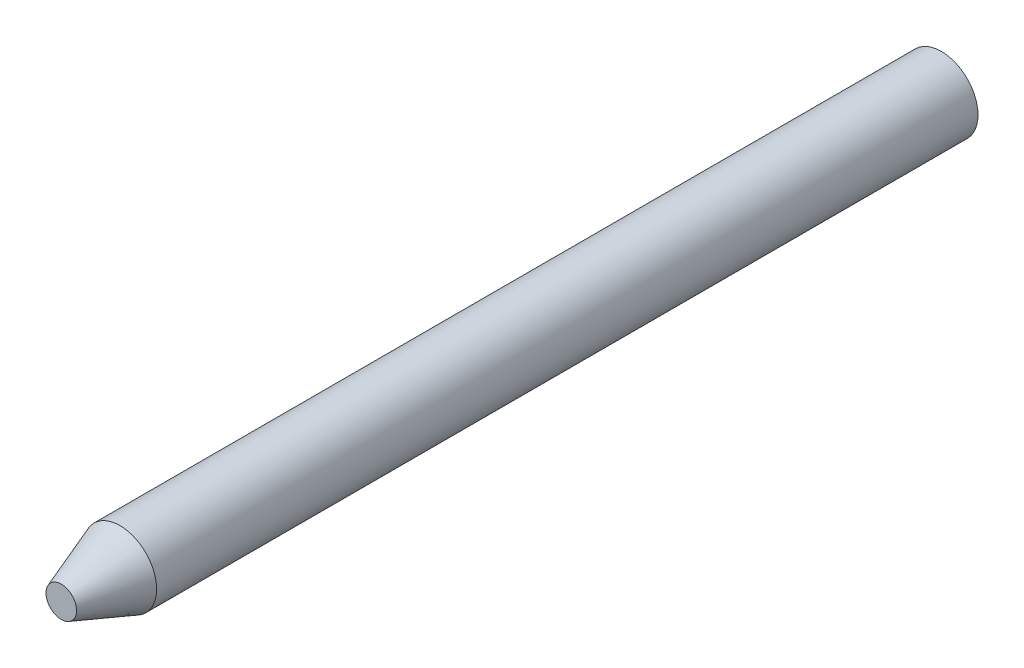
from build123d import *

# Parameters (mm, degrees)
SKETCH_1_R      = 1.25
EXTRUDE_1_DEPTH = 30
CHAMFER_1_SIZE  = 2
CHAMFER_1_SIZE2 = 0.727940469


with BuildPart() as part:
    # 草图1 → 凸台-拉伸1 (new body)
    with BuildSketch(Plane.XY):
        Circle(SKETCH_1_R)
    extrude(amount=EXTRUDE_1_DEPTH)

    # 倒角1
    chamfer_1_edges = [part.edges().sort_by_distance(p)[0] for p in [
        (-1.25, 0, 30),
    ]]
    chamfer_1_side = [part.faces().sort_by_distance(p)[0] for p in [
        (-1.25, 0, 15),
    ]]
    chamfer(chamfer_1_edges, length=CHAMFER_1_SIZE, length2=CHAMFER_1_SIZE2, reference=chamfer_1_side[0])


solid = part.part
